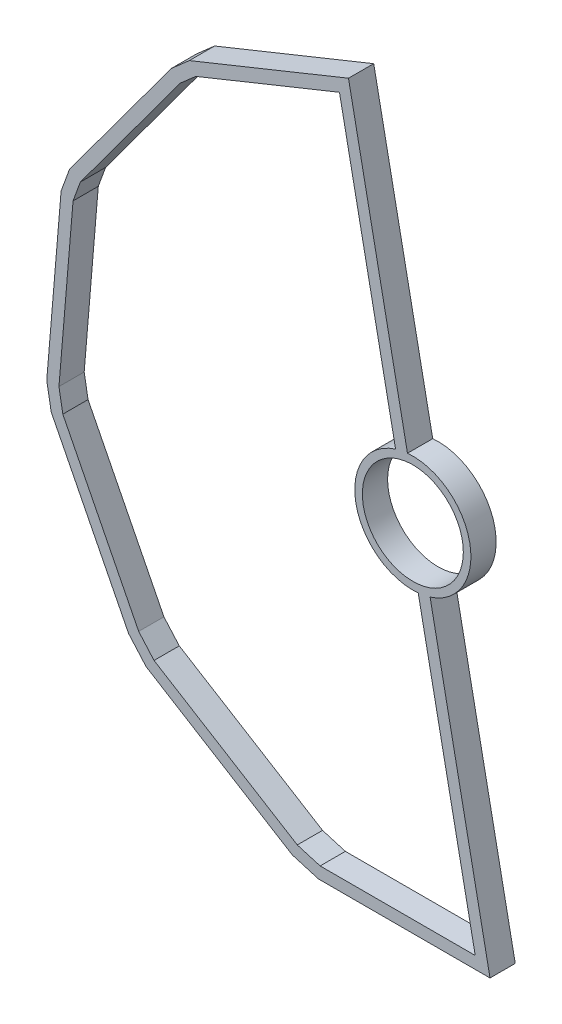
from build123d import *

# Parameters (mm, degrees)
EXTRUDE_1_DEPTH     = 12.5
SKETCH_3_R          = 50
CUT_EXTRUDE_1_DEPTH = 40
SKETCH_4_R          = 57.5
SKETCH_4_R_2        = 50
EXTRUDE_2_DEPTH     = 25


with BuildPart() as part:
    # 草图1 → 凸台-拉伸1 (new, symmetric)
    with BuildSketch(Plane.XY):
        Polygon((10, -352), (85, -352), (-55.185850126, 349.743250156), (-124.732421354, 321.644611463), (-143.278173681, 314.151641145), (-212.824744909, 286.053002452), (-230.575847037, 270.460540253), (-275.085451102, 210.089181938), (-286.954678853, 193.990153053), (-331.464282918, 133.618794737), (-339.828804089, 110.704991943), (-346.104895164, 35.965016687), (-347.77851945, 16.034356619), (-354.054610525, -58.705618637), (-349.658052524, -83.739847979), (-315.841631523, -150.684982948), (-306.823919256, -168.53701894), (-273.007498256, -235.482153909), (-255.615985839, -255.285391269), (-191.736179852, -294.58451012), (-174.701564922, -305.064275147), (-110.821758935, -344.363393998), (-85, -352), (-10, -352), align=None)
        Polygon((-138.78289456, 303.02543489), (-206.438031879, 275.690985101), (-221.684684581, 262.298416336), (-265.426725534, 202.968155298), (-277.295953285, 186.869126414), (-320.782842839, 127.884944314), (-328.005353759, 108.099568976), (-334.146980853, 34.960882567), (-335.820605139, 15.030222499), (-341.966631122, -58.160848878), (-338.146174396, -79.914727665), (-305.130601702, -145.27445246), (-296.112889435, -163.126488451), (-262.984300248, -228.709947873), (-247.790635751, -246.010556193), (-185.448348981, -284.36378691), (-168.413734051, -294.843551937), (-105.890836047, -333.307895427), (-83.26273254, -340), (-10, -340), (10, -340), (70.365682758, -340), (-64.116651933, 333.192555096), (-120.237142233, 310.518405208), align=None, mode=Mode.SUBTRACT)
    extrude(amount=EXTRUDE_1_DEPTH, both=True)

    # 草图3 → 切除-拉伸1 (cut)
    with BuildSketch(Plane.XY.offset(12.5)):
        with Locations((8.563111146, 0)):
            Circle(SKETCH_3_R)
    extrude(amount=-CUT_EXTRUDE_1_DEPTH, mode=Mode.SUBTRACT)

    # 草图4 → 凸台-拉伸2 (add)
    with BuildSketch(Plane.XY.offset(12.5)):
        with Locations((8.563111146, 0)):
            Circle(SKETCH_4_R)
        with Locations((8.563111146, 0)):
            Circle(SKETCH_4_R_2, mode=Mode.SUBTRACT)
    extrude(amount=-EXTRUDE_2_DEPTH)


solid = part.part
